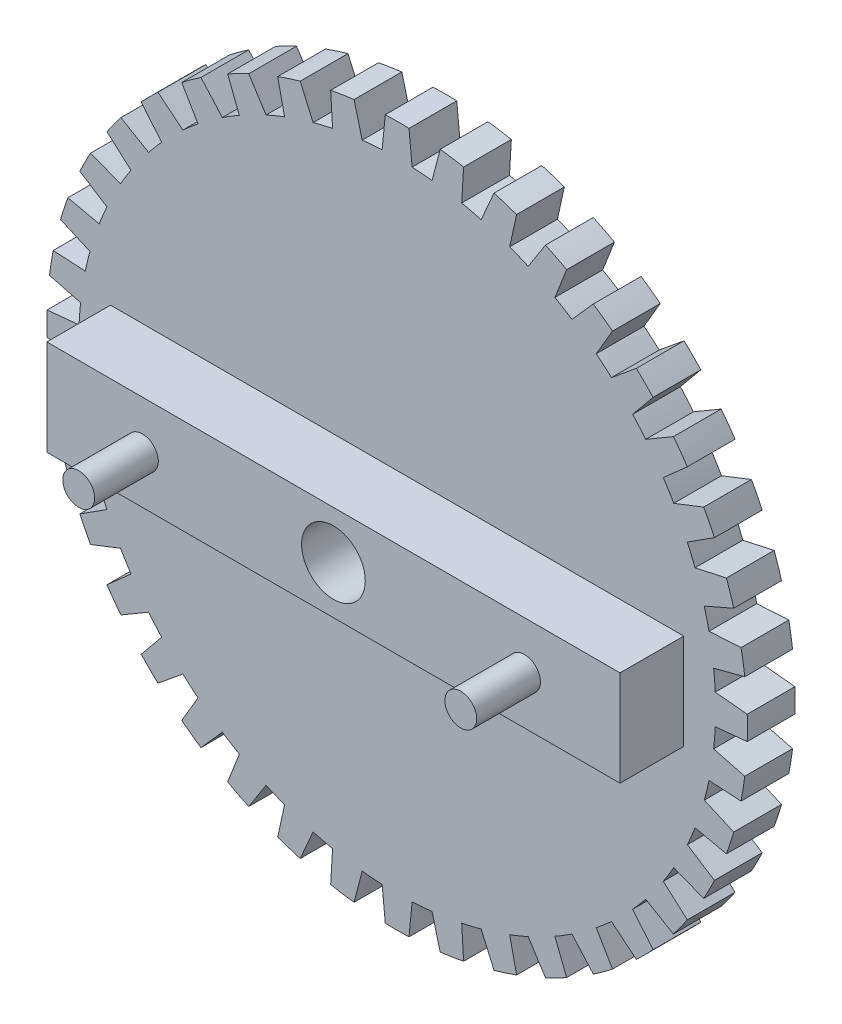
SolidWorks part; units mm, degrees
ref_plane "Front Plane" through (0, 0, 0) normal (0, 0, 1) x (1, 0, 0)
ref_plane "Top Plane" through (0, 0, 0) normal (0, 1, 0) x (1, 0, 0)
ref_plane "Right Plane" through (0, 0, 0) normal (1, 0, 0) x (0, 0, -1)
other "Configuration Table"
sketch "Sketch2" plane through (0, 0, 0) normal (0, 0, 1) x (1, 0, 0)
  line L0 (3.7221, 189.937) -> (4.7076, 179.8891)
  line L1 (-3.7221, 189.937) -> (-4.7076, 179.8891)
  line L2 (0, 0) -> (0, 280.4541) construction
  line L3 (20.8742, 188.0012) -> (20.2758, 177.9229)
  line L4 (13.5217, 189.1658) -> (10.9764, 179.3958)
  line L5 (37.5123, 183.4061) -> (35.3447, 173.5455)
  line L6 (30.4325, 185.7065) -> (26.3902, 176.455)
  line L7 (53.2268, 176.2648) -> (49.5433, 166.8646)
  line L8 (46.594, 179.6444) -> (41.1542, 171.1391)
  line L9 (67.6306, 166.7531) -> (62.5219, 158.0449)
  line L10 (61.6081, 171.1287) -> (54.9048, 163.5791)
  line L11 (80.3691, 155.1053) -> (73.9611, 147.3035)
  line L12 (75.1053, 160.3691) -> (67.3035, 153.9611)
  line L13 (91.1287, 141.6081) -> (83.5791, 134.9048)
  line L14 (86.7531, 147.6306) -> (78.0449, 142.5219)
  line L15 (99.6444, 126.594) -> (91.1391, 121.1542)
  line L16 (96.2648, 133.2268) -> (86.8646, 129.5433)
  line L17 (105.7065, 110.4325) -> (96.455, 106.3902)
  line L18 (103.4061, 117.5123) -> (93.5455, 115.3447)
  line L19 (109.1658, 93.5217) -> (99.3958, 90.9764)
  line L20 (108.0012, 100.8742) -> (97.9229, 100.2758)
  line L21 (109.937, 76.2779) -> (99.8891, 75.2924)
  line L22 (109.937, 83.7221) -> (99.8891, 84.7076)
  line L23 (108.0012, 59.1258) -> (97.9229, 59.7242)
  line L24 (109.1658, 66.4783) -> (99.3958, 69.0236)
  line L25 (103.4061, 42.4877) -> (93.5455, 44.6553)
  line L26 (105.7065, 49.5675) -> (96.455, 53.6098)
  line L27 (96.2648, 26.7732) -> (86.8646, 30.4567)
  line L28 (99.6444, 33.406) -> (91.1391, 38.8458)
  line L29 (86.7531, 12.3694) -> (78.0449, 17.4781)
  line L30 (91.1287, 18.3919) -> (83.5791, 25.0952)
  line L31 (75.1053, -0.3691) -> (67.3035, 6.0389)
  line L32 (80.3691, 4.8947) -> (73.9611, 12.6965)
  line L33 (61.6081, -11.1287) -> (54.9048, -3.5791)
  line L34 (67.6306, -6.7531) -> (62.5219, 1.9551)
  line L35 (46.594, -19.6444) -> (41.1542, -11.1391)
  line L36 (53.2268, -16.2648) -> (49.5433, -6.8646)
  line L37 (30.4325, -25.7065) -> (26.3902, -16.455)
  line L38 (37.5123, -23.4061) -> (35.3447, -13.5455)
  line L39 (13.5217, -29.1658) -> (10.9764, -19.3958)
  line L40 (20.8742, -28.0012) -> (20.2758, -17.9229)
  line L41 (-3.7221, -29.937) -> (-4.7076, -19.8891)
  line L42 (3.7221, -29.937) -> (4.7076, -19.8891)
  line L43 (-20.8742, -28.0012) -> (-20.2758, -17.9229)
  line L44 (-13.5217, -29.1658) -> (-10.9764, -19.3958)
  line L45 (-37.5123, -23.4061) -> (-35.3447, -13.5455)
  line L46 (-30.4325, -25.7065) -> (-26.3902, -16.455)
  line L47 (-53.2268, -16.2648) -> (-49.5433, -6.8646)
  line L48 (-46.594, -19.6444) -> (-41.1542, -11.1391)
  line L49 (-67.6306, -6.7531) -> (-62.5219, 1.9551)
  line L50 (-61.6081, -11.1287) -> (-54.9048, -3.5791)
  line L51 (-80.3691, 4.8947) -> (-73.9611, 12.6965)
  line L52 (-75.1053, -0.3691) -> (-67.3035, 6.0389)
  line L53 (-91.1287, 18.3919) -> (-83.5791, 25.0952)
  line L54 (-86.7531, 12.3694) -> (-78.0449, 17.4781)
  line L55 (-99.6444, 33.406) -> (-91.1391, 38.8458)
  line L56 (-96.2648, 26.7732) -> (-86.8646, 30.4567)
  line L57 (-105.7065, 49.5675) -> (-96.455, 53.6098)
  line L58 (-103.4061, 42.4877) -> (-93.5455, 44.6553)
  line L59 (-109.1658, 66.4783) -> (-99.3958, 69.0236)
  line L60 (-108.0012, 59.1258) -> (-97.9229, 59.7242)
  line L61 (-109.937, 83.7221) -> (-99.8891, 84.7076)
  line L62 (-109.937, 76.2779) -> (-99.8891, 75.2924)
  line L63 (-108.0012, 100.8742) -> (-97.9229, 100.2758)
  line L64 (-109.1658, 93.5217) -> (-99.3958, 90.9764)
  line L65 (-103.4061, 117.5123) -> (-93.5455, 115.3447)
  line L66 (-105.7065, 110.4325) -> (-96.455, 106.3902)
  line L67 (-96.2648, 133.2268) -> (-86.8646, 129.5433)
  line L68 (-99.6444, 126.594) -> (-91.1391, 121.1542)
  line L69 (-86.7531, 147.6306) -> (-78.0449, 142.5219)
  line L70 (-91.1287, 141.6081) -> (-83.5791, 134.9048)
  line L71 (-75.1053, 160.3691) -> (-67.3035, 153.9611)
  line L72 (-80.3691, 155.1053) -> (-73.9611, 147.3035)
  line L73 (-61.6081, 171.1287) -> (-54.9048, 163.5791)
  line L74 (-67.6306, 166.7531) -> (-62.5219, 158.0449)
  line L75 (-46.594, 179.6444) -> (-41.1542, 171.1391)
  line L76 (-53.2268, 176.2648) -> (-49.5433, 166.8646)
  line L77 (-30.4325, 185.7065) -> (-26.3902, 176.455)
  line L78 (-37.5123, 183.4061) -> (-35.3447, 173.5455)
  line L79 (-13.5217, 189.1658) -> (-10.9764, 179.3958)
  line L80 (-20.8742, 188.0012) -> (-20.2758, 177.9229)
  arc A0 (3.7221, 189.937) -> (-3.7221, 189.937) centre (0, 80) ccw
  arc A1 (-4.7076, 179.8891) -> (-10.9764, 179.3958) centre (0, 80) ccw
  arc A2 (20.8742, 188.0012) -> (13.5217, 189.1658) centre (0, 80) ccw
  arc A3 (37.5123, 183.4061) -> (30.4325, 185.7065) centre (0, 80) ccw
  arc A4 (53.2268, 176.2648) -> (46.594, 179.6444) centre (0, 80) ccw
  arc A5 (67.6306, 166.7531) -> (61.6081, 171.1287) centre (0, 80) ccw
  arc A6 (80.3691, 155.1053) -> (75.1053, 160.3691) centre (0, 80) ccw
  arc A7 (91.1287, 141.6081) -> (86.7531, 147.6306) centre (0, 80) ccw
  arc A8 (99.6444, 126.594) -> (96.2648, 133.2268) centre (0, 80) ccw
  arc A9 (105.7065, 110.4325) -> (103.4061, 117.5123) centre (0, 80) ccw
  arc A10 (109.1658, 93.5217) -> (108.0012, 100.8742) centre (0, 80) ccw
  arc A11 (109.937, 76.2779) -> (109.937, 83.7221) centre (0, 80) ccw
  arc A12 (108.0012, 59.1258) -> (109.1658, 66.4783) centre (0, 80) ccw
  arc A13 (103.4061, 42.4877) -> (105.7065, 49.5675) centre (0, 80) ccw
  arc A14 (96.2648, 26.7732) -> (99.6444, 33.406) centre (0, 80) ccw
  arc A15 (86.7531, 12.3694) -> (91.1287, 18.3919) centre (0, 80) ccw
  arc A16 (75.1053, -0.3691) -> (80.3691, 4.8947) centre (0, 80) ccw
  arc A17 (61.6081, -11.1287) -> (67.6306, -6.7531) centre (0, 80) ccw
  arc A18 (46.594, -19.6444) -> (53.2268, -16.2648) centre (0, 80) ccw
  arc A19 (30.4325, -25.7065) -> (37.5123, -23.4061) centre (0, 80) ccw
  arc A20 (13.5217, -29.1658) -> (20.8742, -28.0012) centre (0, 80) ccw
  arc A21 (-3.7221, -29.937) -> (3.7221, -29.937) centre (0, 80) ccw
  arc A22 (-20.8742, -28.0012) -> (-13.5217, -29.1658) centre (0, 80) ccw
  arc A23 (-37.5123, -23.4061) -> (-30.4325, -25.7065) centre (0, 80) ccw
  arc A24 (-53.2268, -16.2648) -> (-46.594, -19.6444) centre (0, 80) ccw
  arc A25 (-67.6306, -6.7531) -> (-61.6081, -11.1287) centre (0, 80) ccw
  arc A26 (-80.3691, 4.8947) -> (-75.1053, -0.3691) centre (0, 80) ccw
  arc A27 (-91.1287, 18.3919) -> (-86.7531, 12.3694) centre (0, 80) ccw
  arc A28 (-99.6444, 33.406) -> (-96.2648, 26.7732) centre (0, 80) ccw
  arc A29 (-105.7065, 49.5675) -> (-103.4061, 42.4877) centre (0, 80) ccw
  arc A30 (-109.1658, 66.4783) -> (-108.0012, 59.1258) centre (0, 80) ccw
  arc A31 (-109.937, 83.7221) -> (-109.937, 76.2779) centre (0, 80) ccw
  arc A32 (-108.0012, 100.8742) -> (-109.1658, 93.5217) centre (0, 80) ccw
  arc A33 (-103.4061, 117.5123) -> (-105.7065, 110.4325) centre (0, 80) ccw
  arc A34 (-96.2648, 133.2268) -> (-99.6444, 126.594) centre (0, 80) ccw
  arc A35 (-86.7531, 147.6306) -> (-91.1287, 141.6081) centre (0, 80) ccw
  arc A36 (-75.1053, 160.3691) -> (-80.3691, 155.1053) centre (0, 80) ccw
  arc A37 (-61.6081, 171.1287) -> (-67.6306, 166.7531) centre (0, 80) ccw
  arc A38 (-46.594, 179.6444) -> (-53.2268, 176.2648) centre (0, 80) ccw
  arc A39 (-30.4325, 185.7065) -> (-37.5123, 183.4061) centre (0, 80) ccw
  arc A40 (-13.5217, 189.1658) -> (-20.8742, 188.0012) centre (0, 80) ccw
  arc A41 (10.9764, 179.3958) -> (4.7076, 179.8891) centre (0, 80) ccw
  arc A42 (26.3902, 176.455) -> (20.2758, 177.9229) centre (0, 80) ccw
  arc A43 (41.1542, 171.1391) -> (35.3447, 173.5455) centre (0, 80) ccw
  arc A44 (54.9048, 163.5791) -> (49.5433, 166.8646) centre (0, 80) ccw
  arc A45 (67.3035, 153.9611) -> (62.5219, 158.0449) centre (0, 80) ccw
  arc A46 (78.0449, 142.5219) -> (73.9611, 147.3035) centre (0, 80) ccw
  arc A47 (86.8646, 129.5433) -> (83.5791, 134.9048) centre (0, 80) ccw
  arc A48 (93.5455, 115.3447) -> (91.1391, 121.1542) centre (0, 80) ccw
  arc A49 (97.9229, 100.2758) -> (96.455, 106.3902) centre (0, 80) ccw
  arc A50 (99.8891, 84.7076) -> (99.3958, 90.9764) centre (0, 80) ccw
  arc A51 (99.3958, 69.0236) -> (99.8891, 75.2924) centre (0, 80) ccw
  arc A52 (96.455, 53.6098) -> (97.9229, 59.7242) centre (0, 80) ccw
  arc A53 (91.1391, 38.8458) -> (93.5455, 44.6553) centre (0, 80) ccw
  arc A54 (83.5791, 25.0952) -> (86.8646, 30.4567) centre (0, 80) ccw
  arc A55 (73.9611, 12.6965) -> (78.0449, 17.4781) centre (0, 80) ccw
  arc A56 (62.5219, 1.9551) -> (67.3035, 6.0389) centre (0, 80) ccw
  arc A57 (49.5433, -6.8646) -> (54.9048, -3.5791) centre (0, 80) ccw
  arc A58 (35.3447, -13.5455) -> (41.1542, -11.1391) centre (0, 80) ccw
  arc A59 (20.2758, -17.9229) -> (26.3902, -16.455) centre (0, 80) ccw
  arc A60 (4.7076, -19.8891) -> (10.9764, -19.3958) centre (0, 80) ccw
  arc A61 (-10.9764, -19.3958) -> (-4.7076, -19.8891) centre (0, 80) ccw
  arc A62 (-26.3902, -16.455) -> (-20.2758, -17.9229) centre (0, 80) ccw
  arc A63 (-41.1542, -11.1391) -> (-35.3447, -13.5455) centre (0, 80) ccw
  arc A64 (-54.9048, -3.5791) -> (-49.5433, -6.8646) centre (0, 80) ccw
  arc A65 (-67.3035, 6.0389) -> (-62.5219, 1.9551) centre (0, 80) ccw
  arc A66 (-78.0449, 17.4781) -> (-73.9611, 12.6965) centre (0, 80) ccw
  arc A67 (-86.8646, 30.4567) -> (-83.5791, 25.0952) centre (0, 80) ccw
  arc A68 (-93.5455, 44.6553) -> (-91.1391, 38.8458) centre (0, 80) ccw
  arc A69 (-97.9229, 59.7242) -> (-96.455, 53.6098) centre (0, 80) ccw
  arc A70 (-99.8891, 75.2924) -> (-99.3958, 69.0236) centre (0, 80) ccw
  arc A71 (-99.3958, 90.9764) -> (-99.8891, 84.7076) centre (0, 80) ccw
  arc A72 (-96.455, 106.3902) -> (-97.9229, 100.2758) centre (0, 80) ccw
  arc A73 (-91.1391, 121.1542) -> (-93.5455, 115.3447) centre (0, 80) ccw
  arc A74 (-83.5791, 134.9048) -> (-86.8646, 129.5433) centre (0, 80) ccw
  arc A75 (-73.9611, 147.3035) -> (-78.0449, 142.5219) centre (0, 80) ccw
  arc A76 (-62.5219, 158.0449) -> (-67.3035, 153.9611) centre (0, 80) ccw
  arc A77 (-49.5433, 166.8646) -> (-54.9048, 163.5791) centre (0, 80) ccw
  arc A78 (-35.3447, 173.5455) -> (-41.1542, 171.1391) centre (0, 80) ccw
  arc A79 (-20.2758, 177.9229) -> (-26.3902, 176.455) centre (0, 80) ccw
  circle A80 centre (0, 80) radius 10
  point P169 (0, 80)
  dimension "D1" = 40
extrude "Boss-Extrude1" add sketch "Sketch2" along normal blind 15
sketch "Sketch3" plane through (0, 0, 15) normal (0, 0, 1) x (1, 0, 0)
  line L1 (-90, 95) -> (90, 95)
  line L2 (-90, 95) -> (-90, 65)
  line L3 (-90, 65) -> (90, 65)
  line L4 (90, 95) -> (90, 65)
  line L5 (-90, 95) -> (90, 65) construction
  line L6 (-90, 65) -> (90, 95) construction
  circle A0 centre (0, 80) radius 10
  point P0 (0, 80)
  dimension "D1" = 30
  dimension "D2" = 180
extrude "Boss-Extrude2" add sketch "Sketch3" along normal blind 20
sketch "Sketch4" plane through (0, 0, 35) normal (0, 0, 1) x (1, 0, 0)
  line L0 (90, 65) -> (90, 95) construction
  line L1 (0, -19.25) -> (0, 19.25) construction
  circle A0 centre (60, 80) radius 5
  circle A1 centre (-60, 80) radius 5
  dimension "D1" = 30
extrude "Boss-Extrude3" add sketch "Sketch4" along normal blind 20
